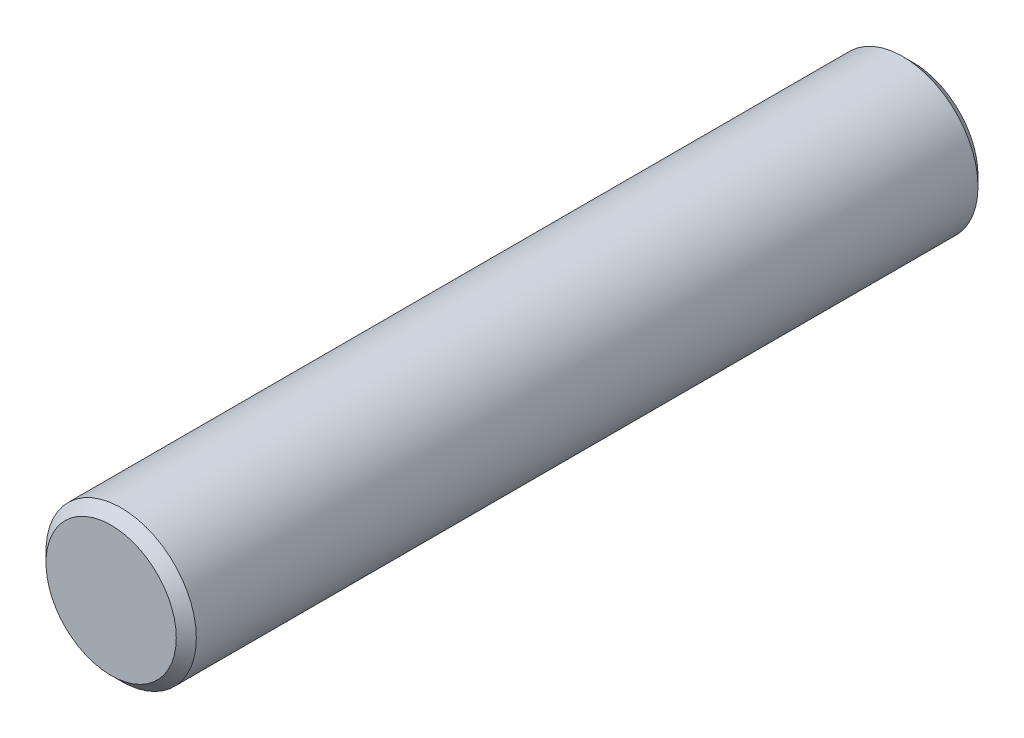
SolidWorks part; units mm, degrees
ref_plane "Front Plane" through (0, 0, 0) normal (0, 0, 1) x (1, 0, 0)
ref_plane "Top Plane" through (0, 0, 0) normal (0, 1, 0) x (1, 0, 0)
ref_plane "Right Plane" through (0, 0, 0) normal (1, 0, 0) x (0, 0, -1)
other "Configuration Table"
sketch "Sketch1" plane through (0, 0, 0) normal (0, 0, 1) x (1, 0, 0)
  circle A0 centre (0, 0) radius 1.5
  dimension "D1" = 3
extrude "Boss-Extrude1" add sketch "Sketch1" along normal blind 16
chamfer "Chamfer1" distance 0.2 angle 45 2 edges at (1.5, 0, 0) (1.5, 0, 16)
